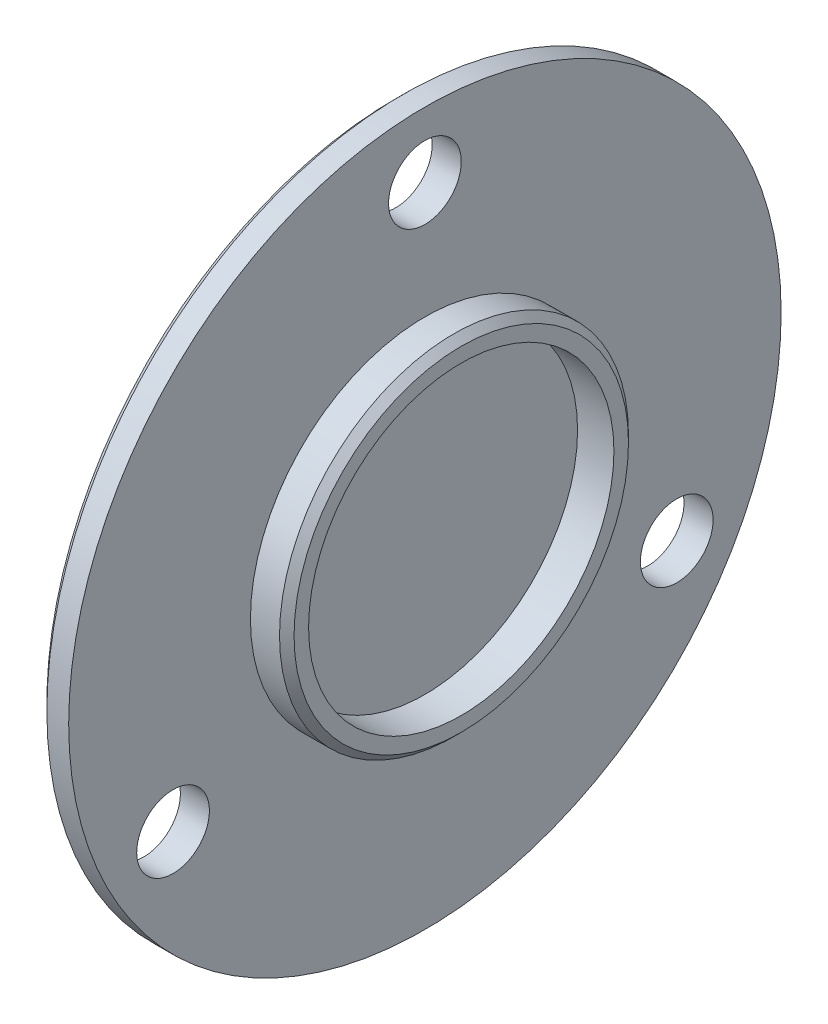
from build123d import *

# Parameters (mm, degrees)
SKETCH1_R               = 24.5
BOSS_EXTRUDE1_DEPTH     = 2
SKETCH2_R               = 12
BOSS_EXTRUDE2_DEPTH     = 2.5
CUT_EXTRUDE1_DEPTH      = 35.939232962
CUT_EXTRUDE1_DEPTH_BACK = 2.5
SKETCH3_R               = 10.5
SKETCH4_R               = 2.5
CUT_EXTRUDE2_DEPTH      = 2.5
CHAMFER1_SIZE           = 0.5


with BuildPart() as part:
    # Sketch1 → Boss-Extrude1 (new body)
    with BuildSketch(Plane(origin=(0, 0, 0), x_dir=(0, 0, -1), z_dir=(1, 0, 0))):
        Circle(SKETCH1_R)
    extrude(amount=BOSS_EXTRUDE1_DEPTH)

    # Sketch2 → Boss-Extrude2 (add)
    with BuildSketch(Plane(origin=(2, 0, 0), x_dir=(0, 0, -1), z_dir=(1, 0, 0))):
        Circle(SKETCH2_R)
    extrude(amount=BOSS_EXTRUDE2_DEPTH)

    # Sketch3 → Cut-Extrude1 (cut, two sides: drawn at the far end of the back side and taken through both)
    with BuildSketch(Plane(origin=(4.5, 0, 0), x_dir=(0, 0, -1), z_dir=(1, 0, 0)).offset(-CUT_EXTRUDE1_DEPTH_BACK)):
        with Locations(Location((0, 0, 0), (0, 0, 180))):
            Circle(SKETCH3_R)
    extrude(amount=CUT_EXTRUDE1_DEPTH + CUT_EXTRUDE1_DEPTH_BACK, mode=Mode.SUBTRACT)

    # Sketch4 → Cut-Extrude2 (cut)
    with BuildSketch(Plane.ZY):
        with Locations((0, 20)):
            Circle(SKETCH4_R)
        with Locations((17.320508076, -10)):
            Circle(SKETCH4_R)
        with Locations((-17.320508076, -10)):
            Circle(SKETCH4_R)
    extrude(amount=-CUT_EXTRUDE2_DEPTH, mode=Mode.SUBTRACT)

    # Chamfer1
    chamfer1_edges = [part.edges().sort_by_distance(p)[0] for p in [
        (0, 0, 24.5),
        (4.5, 0, 12),
    ]]
    chamfer(chamfer1_edges, length=CHAMFER1_SIZE)


solid = part.part
